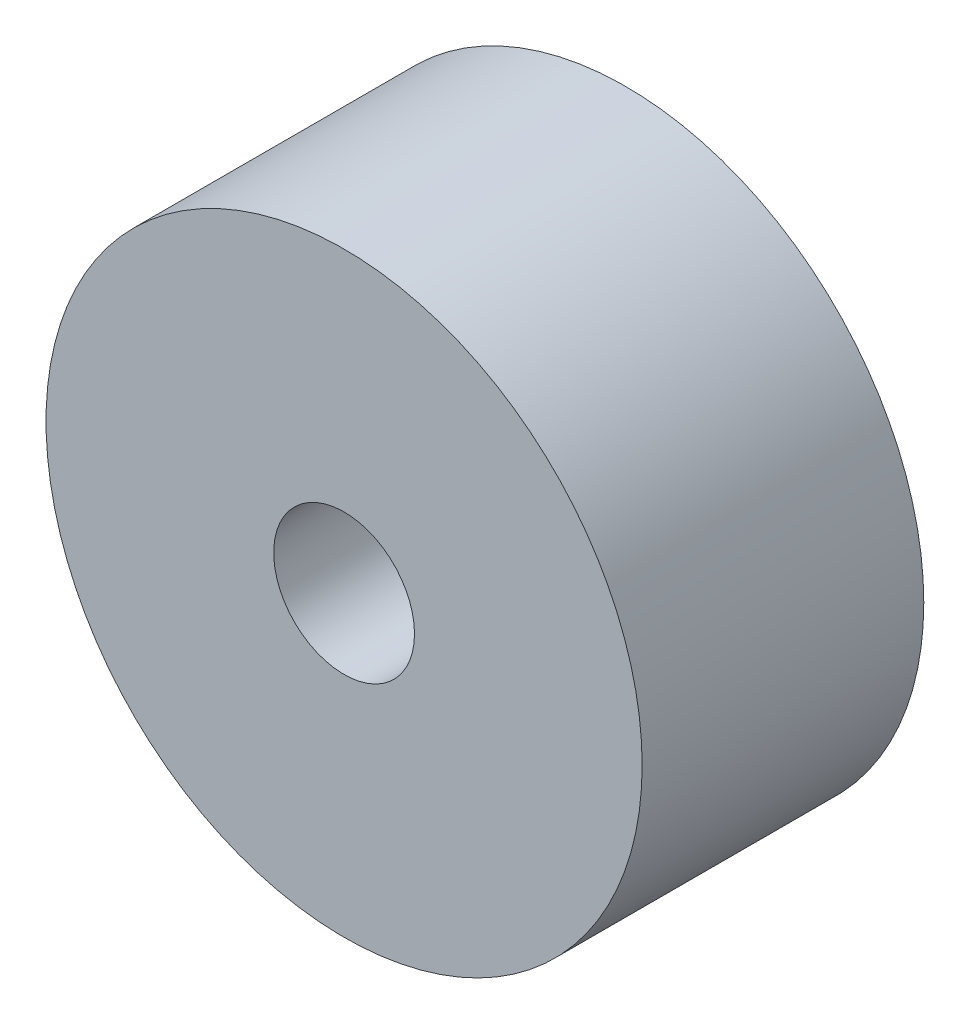
from build123d import *

# Parameters (mm, degrees)
SKETCH1_R           = 12.7
SKETCH1_R_2         = 3
BOSS_EXTRUDE1_DEPTH = 12


with BuildPart() as part:
    # Sketch1 → Boss-Extrude1 (new body)
    with BuildSketch(Plane.XY):
        Circle(SKETCH1_R)
        Circle(SKETCH1_R_2, mode=Mode.SUBTRACT)
    extrude(amount=BOSS_EXTRUDE1_DEPTH)


solid = part.part
